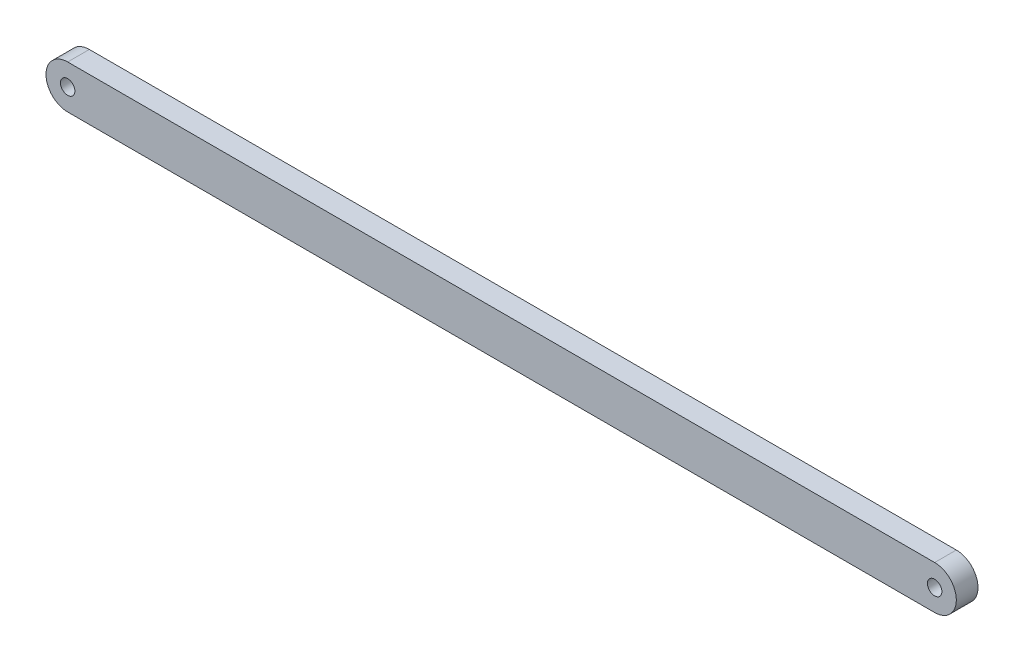
from build123d import *

# Parameters (mm, degrees)
SKETCH_1_R      = 2
EXTRUDE_1_DEPTH = 6


with BuildPart() as part:
    # 草图1 → 凸台-拉伸1 (new body)
    with BuildSketch(Plane.XY):
        with BuildLine():
            Line((-119.735261546, 7.191323041), (120.264738454, 7.191323041))
            ThreePointArc((120.264738454, 7.191323041), (126.264738454, 1.191323041), (120.264738454, -4.808676959))
            Line((120.264738454, -4.808676959), (-119.735261546, -4.808676959))
            ThreePointArc((-119.735261546, -4.808676959), (-125.735261546, 1.191323041), (-119.735261546, 7.191323041))
        make_face()
        with Locations((-119.735261546, 1.191323041)):
            Circle(SKETCH_1_R, mode=Mode.SUBTRACT)
        with Locations((120.264738454, 1.191323041)):
            Circle(SKETCH_1_R, mode=Mode.SUBTRACT)
    extrude(amount=EXTRUDE_1_DEPTH)


solid = part.part
